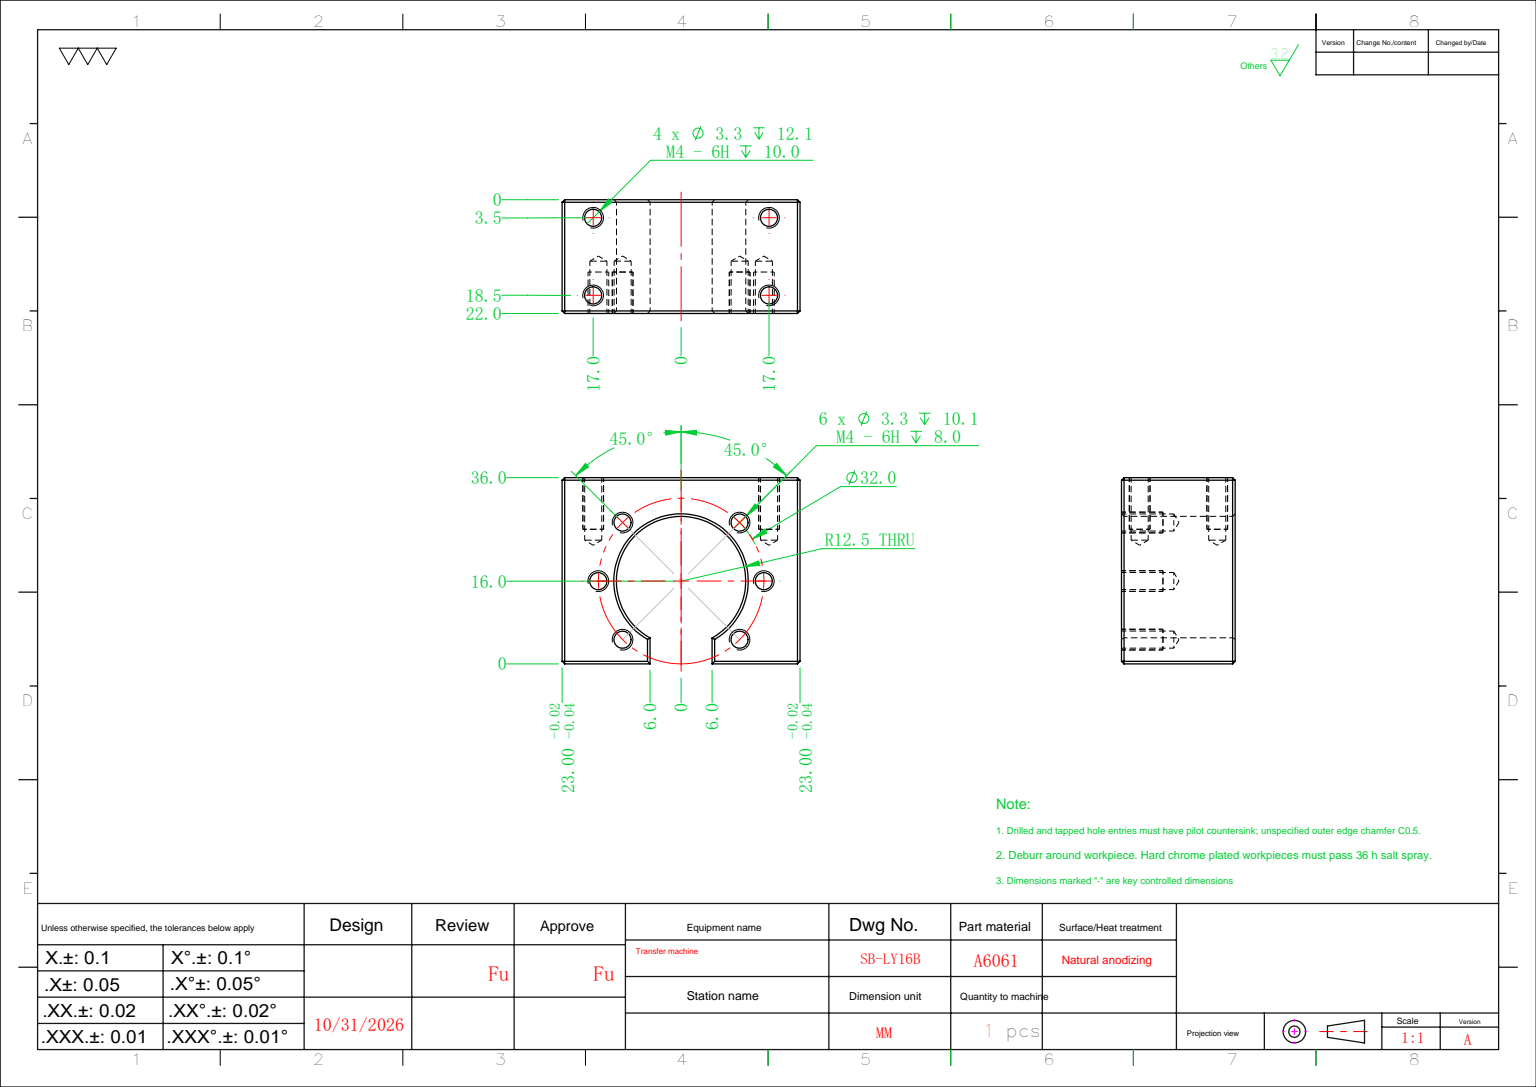
from build123d import *

# Parameters (mm, degrees)
SKETCH_1_W             = 46
SKETCH_1_H             = 36
EXTRUDE_1_DEPTH        = 22
CUT_EXTRUDE_2_DEPTH    = 37.565010598
CHAMFER_1_SIZE         = 0.5
HOLE_WIZARD_M4_1_D     = 3.3
HOLE_WIZARD_M4_1_DEPTH = 12.1
HOLE_WIZARD_M4_1_TIP   = 0.991420021
HOLE_WIZARD_M4_2_D     = 3.3
HOLE_WIZARD_M4_2_DEPTH = 10.1
HOLE_WIZARD_M4_2_TIP   = 0.991420021


with BuildPart() as part:
    # 草图1 → 凸台-拉伸1 (new body)
    with BuildSketch(Plane.XY):
        Rectangle(SKETCH_1_W, SKETCH_1_H)
    extrude(amount=EXTRUDE_1_DEPTH)

    # 草图5 → 切除-拉伸2 (cut, through all)
    with BuildSketch(Plane.XY.offset(22)):
        with BuildLine():
            Line((-6, -12.9658561), (-6, -18))
            Line((-6, -18), (6, -18))
            Line((6, -18), (6, -12.9658561))
            ThreePointArc((6, -12.9658561), (0, 10.5), (-6, -12.9658561))
        make_face()
    extrude(amount=-CUT_EXTRUDE_2_DEPTH, mode=Mode.SUBTRACT)

    # 倒角1
    chamfer_1_edges = [part.edges().sort_by_distance(p)[0] for p in [
        (-23, 0, 22),
        (-14.5, -18, 22),
        (14.5, -18, 0),
        (14.5, -18, 22),
        (0, 10.5, 0),
        (6, -15.48292805, 0),
        (-6, -15.48292805, 0),
        (0, 10.5, 22),
        (-6, -15.48292805, 22),
        (6, -15.48292805, 22),
        (23, 0, 22),
        (-14.5, -18, 0),
        (-23, 0, 0),
        (0, 18, 0),
        (23, 0, 0),
        (0, 18, 22),
        (23, -18, 11),
        (-23, -18, 11),
        (-23, 18, 11),
        (23, 18, 11),
    ]]
    chamfer(chamfer_1_edges, length=CHAMFER_1_SIZE)

    # M4 螺纹孔1
    with Locations(Plane(origin=(0, 18, 0), x_dir=(1, 0, 0), z_dir=(0, 1, 0))):
        with Locations((17, -18.5), (17, -3.5), (-17, -3.5), (-17, -18.5)):
            Hole(HOLE_WIZARD_M4_1_D / 2, depth=HOLE_WIZARD_M4_1_DEPTH)
            with Locations((0, 0, -(HOLE_WIZARD_M4_1_DEPTH + HOLE_WIZARD_M4_1_TIP / 2))):  # 118° drill point
                Cone(0, HOLE_WIZARD_M4_1_D / 2, HOLE_WIZARD_M4_1_TIP, mode=Mode.SUBTRACT)

    # M4 螺纹孔2
    with Locations(Plane(origin=(0, 0, 0), x_dir=(-1, 0, 0), z_dir=(0, 0, -1))):
        with Locations((-16, -2), (-11.313708499, 9.313708499), (11.313708499, 9.313708499), (16, -2), (-11.313708499, -13.313708499), (11.313708499, -13.313708499)):
            Hole(HOLE_WIZARD_M4_2_D / 2, depth=HOLE_WIZARD_M4_2_DEPTH)
            with Locations((0, 0, -(HOLE_WIZARD_M4_2_DEPTH + HOLE_WIZARD_M4_2_TIP / 2))):  # 118° drill point
                Cone(0, HOLE_WIZARD_M4_2_D / 2, HOLE_WIZARD_M4_2_TIP, mode=Mode.SUBTRACT)


solid = part.part
